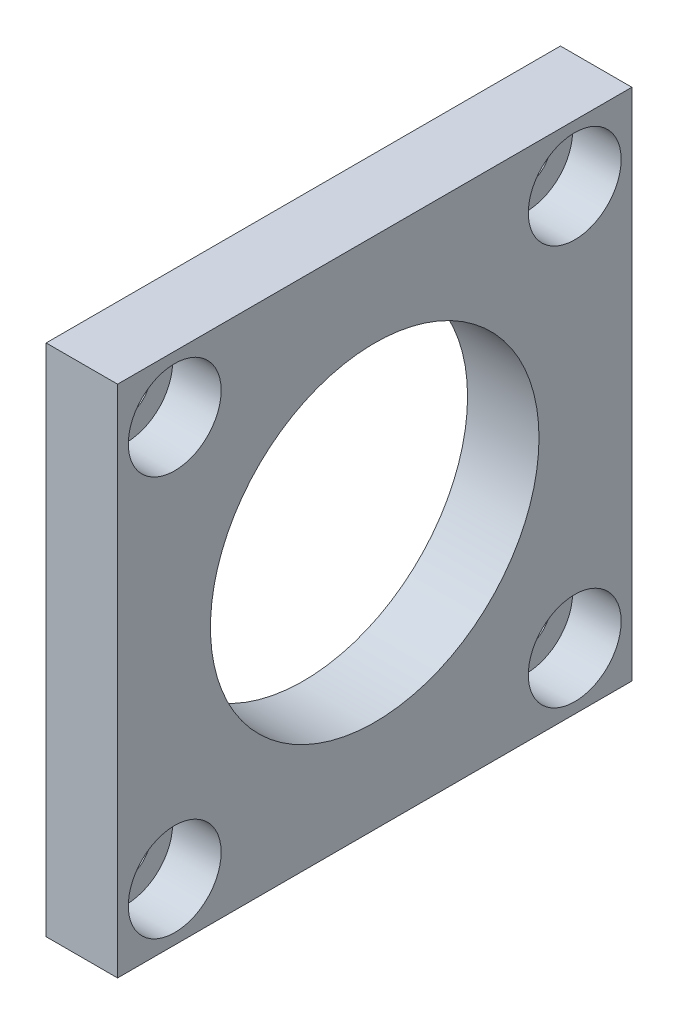
SolidWorks part; units mm, degrees
ref_plane "Front Plane" through (0, 0, 0) normal (0, 0, 1) x (1, 0, 0)
ref_plane "Top Plane" through (0, 0, 0) normal (0, 1, 0) x (1, 0, 0)
ref_plane "Right Plane" through (0, 0, 0) normal (1, 0, 0) x (0, 0, -1)
sketch "Sketch1" plane through (0, 0, 0) normal (1, 0, 0) x (0, 0, -1)
  line L1 (-18, 18) -> (18, 18)
  line L2 (-18, 18) -> (-18, -18)
  line L3 (-18, -18) -> (18, -18)
  line L4 (18, 18) -> (18, -18)
  line L5 (-18, 18) -> (18, -18) construction
  line L6 (-18, -18) -> (18, 18) construction
  point P0 (0, 0)
  dimension "D1" = 36
  dimension "D2" = 36
extrude "Boss-Extrude1" add sketch "Sketch1" along normal mid plane 5
hole_wizard "CBORE for M3 Hex Socket Head Cap Screw1" positions "Sketch3" profile "Sketch4" counterbore size "M3" standard "ISO" end condition through all
sketch "Sketch3" plane through (2.5, 0, 0) normal (1, 0, 0) x (0, 0, -1)
  line L0 (0, 0) -> (20.898, 0) construction
  line L2 (0, 0) -> (0, 24.1488) construction
  point P0 (-14, 14)
  point P2 (14, 14)
  point P4 (-14, -14)
  point P6 (14, -14)
  dimension "D1" = 28
  dimension "D2" = 28
sketch "Sketch4" plane through (2.5, 14, 14) normal (0, 1, 0) x (0, 0, -1)
  line L0 (0, 0) -> (0, 5)
  line L1 (0, 5) -> (1.7, 5)
  line L3 (1.7, 5) -> (1.7, 3.4)
  line L4 (1.7, 3.4) -> (3.25, 3.4)
  line L5 (3.25, 3.4) -> (3.25, 0)
  line L7 (3.25, 0) -> (0, 0)
  line L11 (0, -6.35) -> (0, 107.95) construction
  dimension "通孔孔直径" = 3.4
  dimension "通孔孔深度" = 5
  dimension "柱形沉头孔直径" = 6.5
  dimension "柱形沉头孔深度" = 3.4
sketch "Sketch5" plane through (2.5, 0, 0) normal (1, 0, 0) x (0, 0, -1)
  circle A0 centre (0, 0) radius 11.5
  dimension "D1" = 23
extrude "Cut-Extrude2" cut sketch "Sketch5" against normal through all
